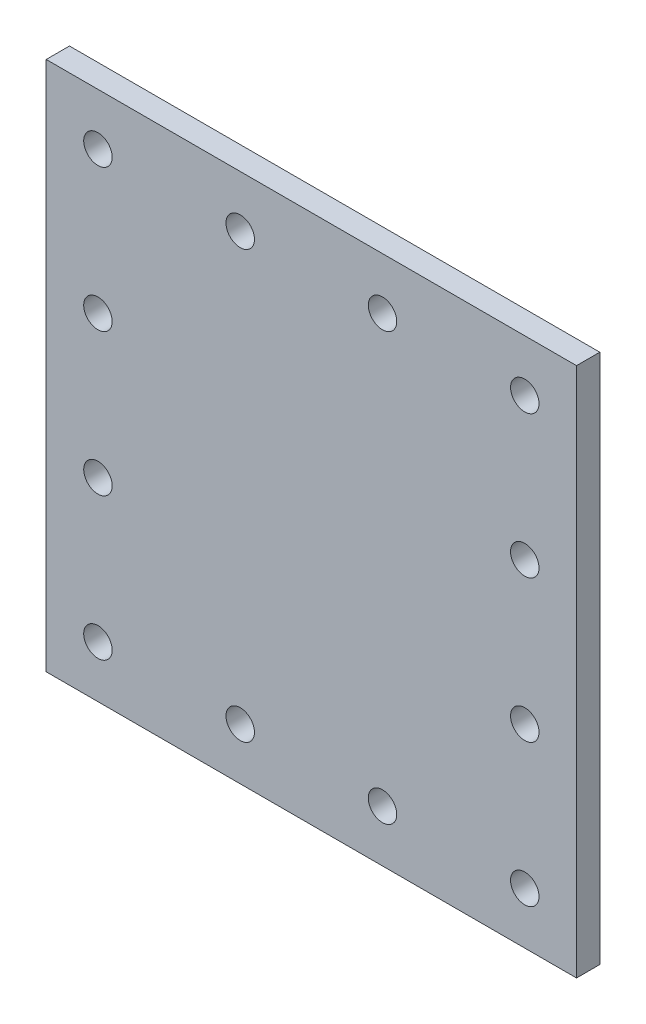
SolidWorks part; units mm, degrees
ref_plane "Front Plane" through (0, 0, 0) normal (0, 0, 1) x (1, 0, 0)
ref_plane "Top Plane" through (0, 0, 0) normal (0, 1, 0) x (1, 0, 0)
ref_plane "Right Plane" through (0, 0, 0) normal (1, 0, 0) x (0, 0, -1)
sketch "Sketch1" plane through (0, 0, 0) normal (0, 0, 1) x (1, 0, 0)
  line L1 (205, 205) -> (-205, 205)
  line L2 (205, 205) -> (205, -205)
  line L3 (205, -205) -> (-205, -205)
  line L4 (-205, 205) -> (-205, -205)
  line L5 (205, 205) -> (-205, -205) construction
  line L6 (205, -205) -> (-205, 205) construction
  point P0 (0, 0)
  dimension "D1" = 410
  dimension "D2" = 410
extrude "Boss-Extrude1" add sketch "Sketch1" along normal blind 18
sketch "Sketch2" plane through (0, 0, 18) normal (0, 0, 1) x (1, 0, 0)
  line L1 (165, 165) -> (-165, 165) construction
  line L2 (165, 165) -> (165, -165) construction
  line L3 (165, -165) -> (-165, -165) construction
  line L4 (-165, 165) -> (-165, -165) construction
  line L5 (165, 165) -> (-165, -165) construction
  line L6 (165, -165) -> (-165, 165) construction
  circle A0 centre (-165, 165) radius 11
  circle A1 centre (165, 165) radius 11
  circle A2 centre (165, -165) radius 11
  circle A3 centre (-165, -165) radius 11
  circle A4 centre (-165, 55) radius 11
  circle A5 centre (-165, -55) radius 11
  circle A6 centre (-55, 165) radius 11
  circle A7 centre (55, 165) radius 11
  circle A8 centre (165, 55) radius 11
  circle A9 centre (165, -55) radius 11
  circle A10 centre (-55, -165) radius 11
  circle A11 centre (55, -165) radius 11
  point P0 (0, 0)
  dimension "D3" = 22
  dimension "D4" = 22
  dimension "D1" = 330
  dimension "D2" = 330
  dimension "D5" = 110
  dimension "D6" = 110
  dimension "D7" = 110
  dimension "D8" = 110
extrude "Cut-Extrude1" cut sketch "Sketch2" against normal blind 18
